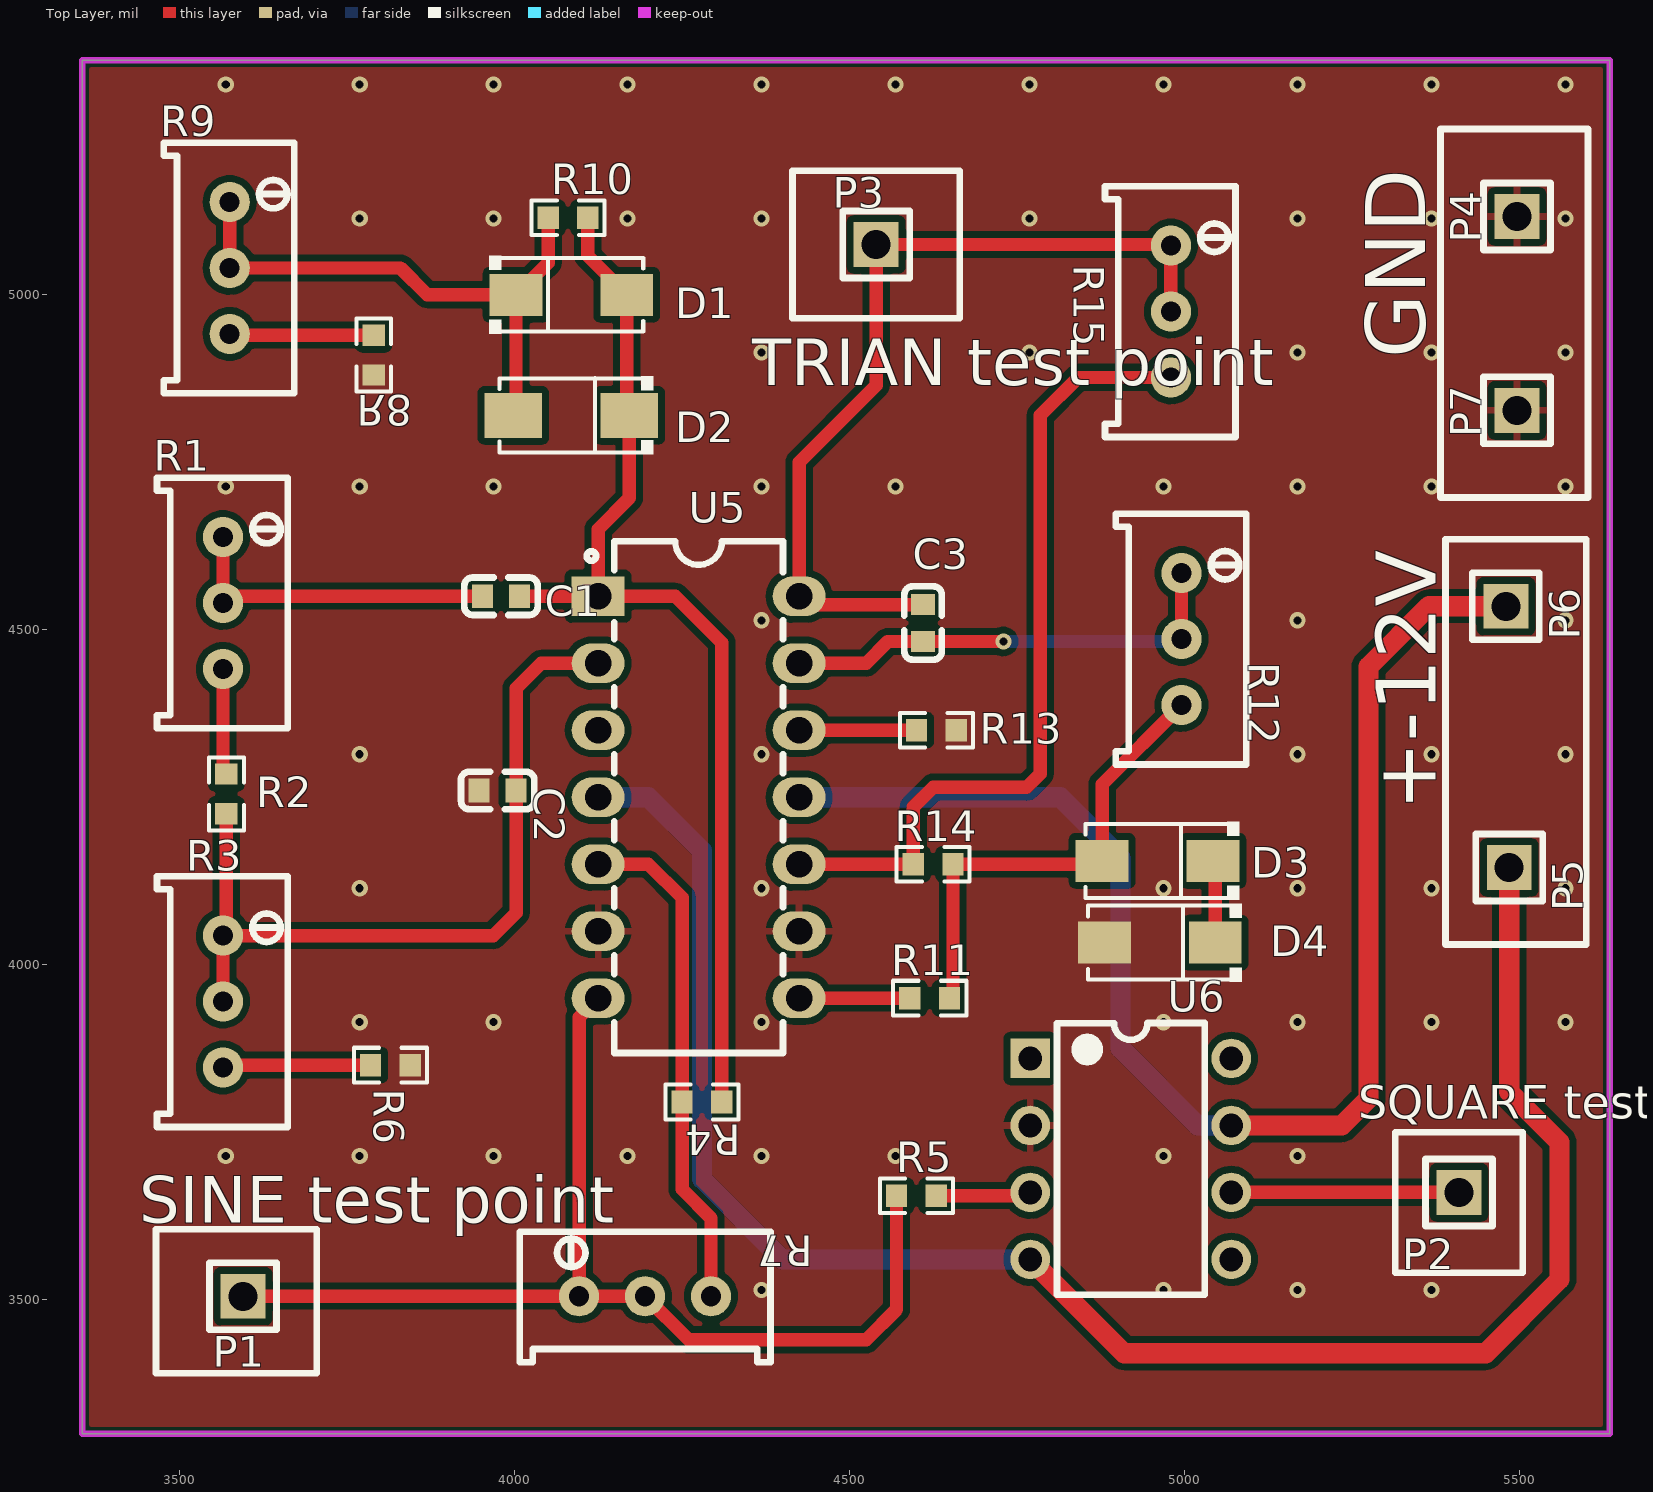
[diagram p0: Top Layer view]
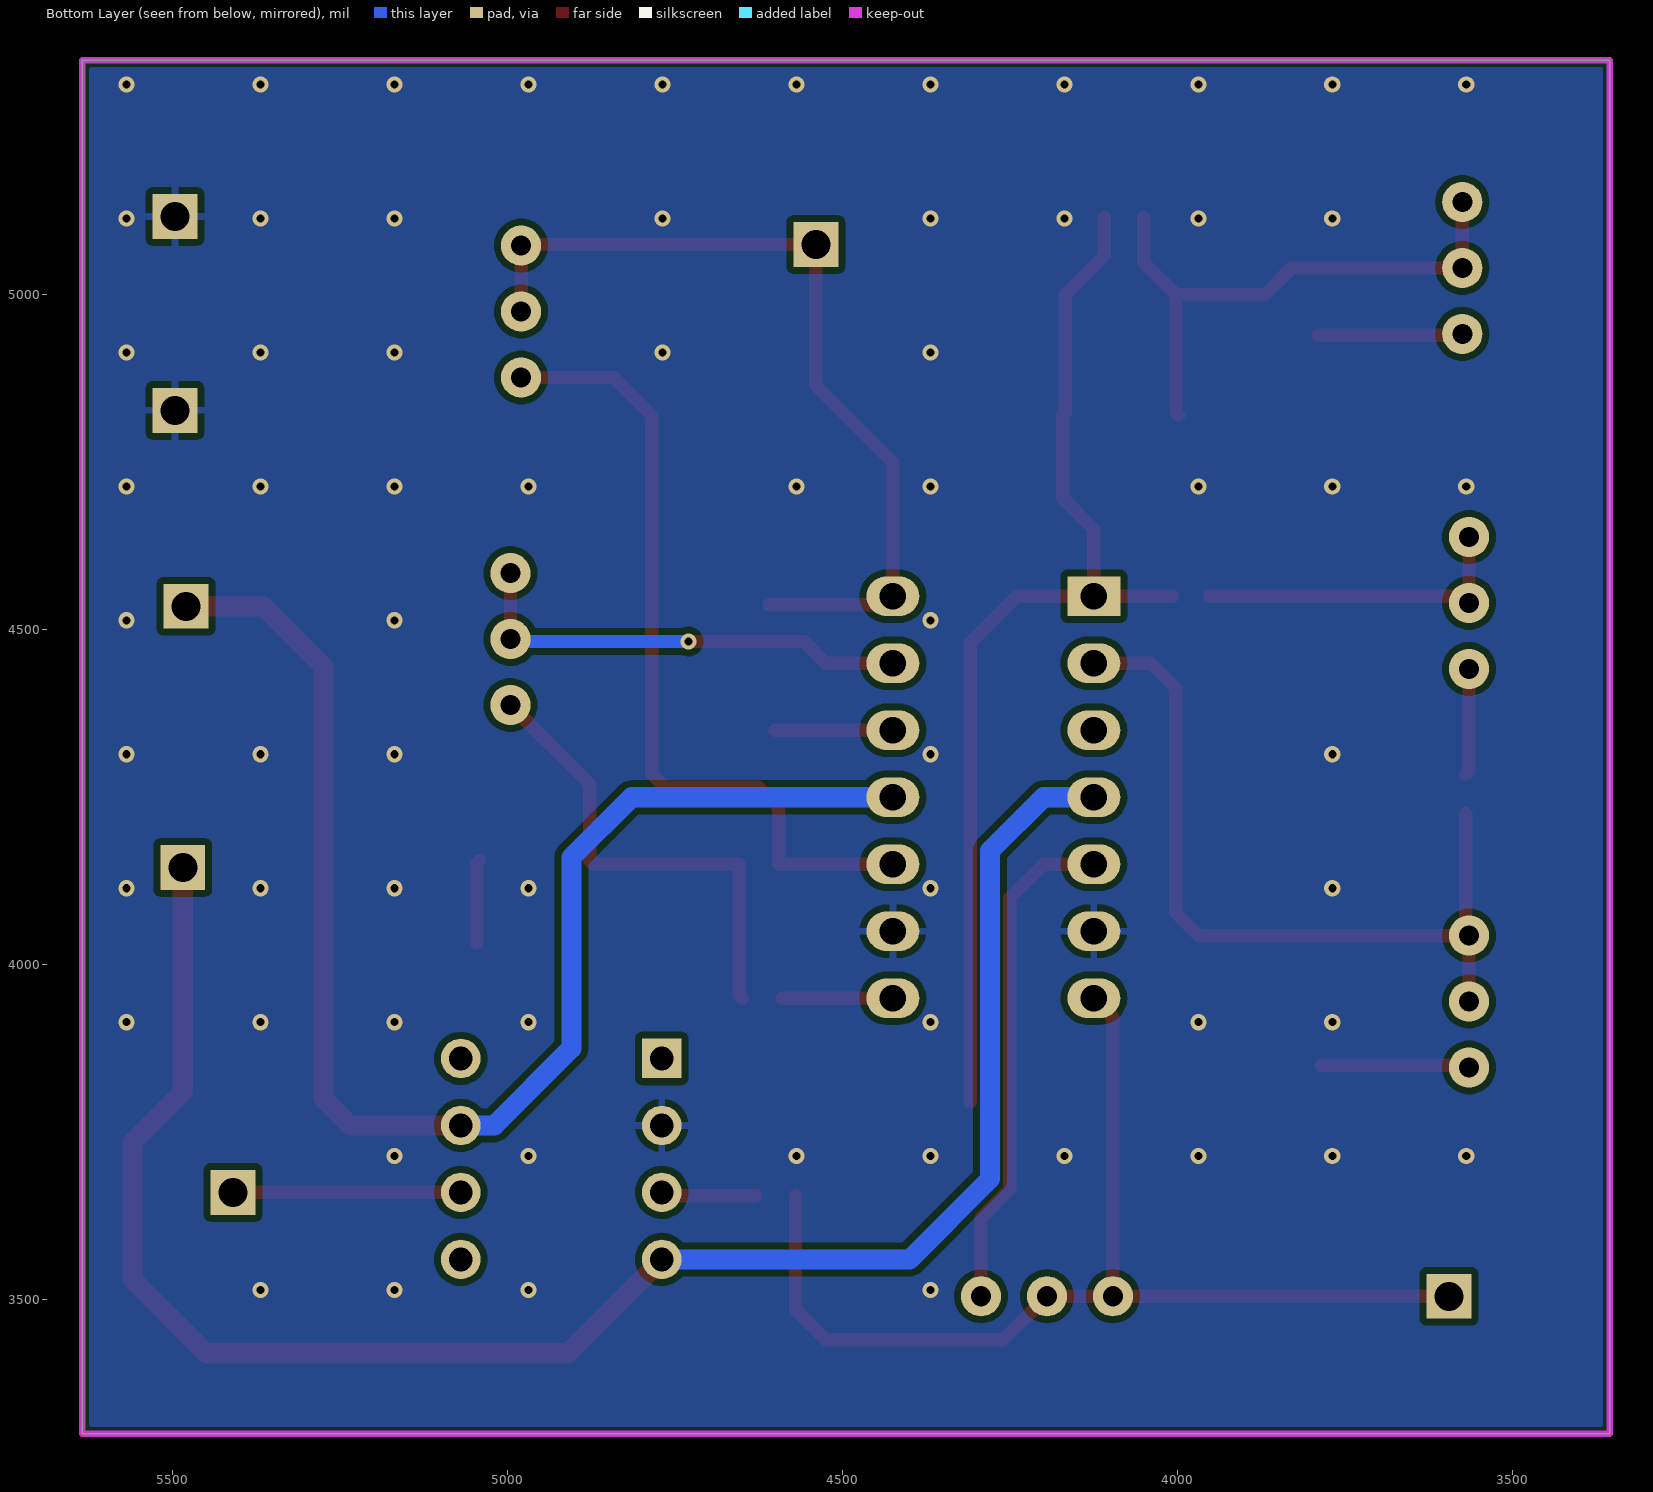
[diagram p1: Bottom Layer view, seen from below]
# Altium PCB MISC51008.pcbdoc
Units mil, origin at the board's own origin, x right, y up, seen from the top; angles counter-clockwise.
Board outline 2280 x 2050 mil, 2 copper layers (Top Layer, Bottom Layer), stack 62.206 mil thick; 31 components, 21 nets, 79 pads, 67 vias.

## Layer stack, top to bottom
Top Solder Mask Layer: solder mask 0.394, Dk 3.3
Top Layer: signal copper 1.379
Dielectric1: surface 59.449, FR4, Dk 4.5
Bottom Layer: signal copper 1.378
Bottom Solder Mask Layer: solder mask 0.394, Dk 3.3

## Board outline
3355,5350 3355,3300 5635,3300 5635,5350

## Design rules (kind name [scope] priority, off if disabled: settings)
BoardOutlineClearance copperThickness2oz_1 [All] p2 off: genericclearance=7.99 ignorepadtopadclearanceinfootprint=FALSE except(0: Arc-SplitContinuation Track-SplitContinuation SMDPad-SplitContinuation THPad-SplitContinuation Via-SplitContinuation Fill-SplitContinuation Region-SplitContinuation Poly-SplitContinuation Text-SplitContinuation Hole-SplitContinuation; 5.98: Arc-CutoutEdge SMDPad-CutoutEdge THPad-CutoutEdge Via-CutoutEdge Fill-CutoutEdge Region-CutoutEdge Text-CutoutEdge; 6.93: Hole-OutlineEdge Hole-CutoutEdge; 10: Poly-OutlineEdge Poly-CutoutEdge; 11.81: Arc-OutlineEdge Track-OutlineEdge SMDPad-OutlineEdge THPad-OutlineEdge Via-OutlineEdge Fill-OutlineEdge Region-OutlineEdge Text-OutlineEdge Track-CutoutEdge)
BoardOutlineClearance Plane_innerPlane_1 [All] p4 off: genericclearance=4.02 ignorepadtopadclearanceinfootprint=FALSE except(0: Arc-SplitContinuation Track-SplitContinuation SMDPad-SplitContinuation THPad-SplitContinuation Via-SplitContinuation Fill-SplitContinuation Region-SplitContinuation Poly-SplitContinuation Text-SplitContinuation Hole-SplitContinuation; 5.98: SMDPad-CutoutEdge THPad-CutoutEdge Via-CutoutEdge Fill-CutoutEdge Region-CutoutEdge Text-CutoutEdge; 6.93: Hole-OutlineEdge Hole-CutoutEdge; 10: Poly-OutlineEdge Poly-CutoutEdge; 11.81: Arc-OutlineEdge Track-OutlineEdge SMDPad-OutlineEdge THPad-OutlineEdge Via-OutlineEdge Fill-OutlineEdge Region-OutlineEdge Text-OutlineEdge Arc-CutoutEdge Track-CutoutEdge)
BoardOutlineClearance Copper_copperRegion_1 [All] p6 off: genericclearance=4.02 ignorepadtopadclearanceinfootprint=FALSE except(0: Arc-SplitContinuation Track-SplitContinuation SMDPad-SplitContinuation THPad-SplitContinuation Via-SplitContinuation Fill-SplitContinuation Region-SplitContinuation Poly-SplitContinuation Text-SplitContinuation Hole-SplitContinuation; 5.98: SMDPad-CutoutEdge THPad-CutoutEdge Via-CutoutEdge Fill-CutoutEdge Region-CutoutEdge Text-CutoutEdge; 6.93: Hole-OutlineEdge Hole-CutoutEdge; 10: Poly-OutlineEdge Poly-CutoutEdge; 11.81: Arc-OutlineEdge Track-OutlineEdge SMDPad-OutlineEdge THPad-OutlineEdge Via-OutlineEdge Fill-OutlineEdge Region-OutlineEdge Text-OutlineEdge Arc-CutoutEdge Track-CutoutEdge)
BoardOutlineClearance copperThickness1oz_1 [All] p8: genericclearance=4.02 ignorepadtopadclearanceinfootprint=FALSE except(0: Arc-SplitContinuation Track-SplitContinuation SMDPad-SplitContinuation THPad-SplitContinuation Via-SplitContinuation Fill-SplitContinuation Region-SplitContinuation Poly-SplitContinuation Text-SplitContinuation Hole-SplitContinuation; 5.98: SMDPad-CutoutEdge THPad-CutoutEdge Via-CutoutEdge Fill-CutoutEdge Region-CutoutEdge Text-CutoutEdge; 6.93: Hole-OutlineEdge Hole-CutoutEdge; 10: Poly-OutlineEdge Poly-CutoutEdge; 11.81: Arc-OutlineEdge Track-OutlineEdge SMDPad-OutlineEdge THPad-OutlineEdge Via-OutlineEdge Fill-OutlineEdge Region-OutlineEdge Text-OutlineEdge Arc-CutoutEdge Track-CutoutEdge)
Clearance copperThickness2oz [All] p1 off: gap=7.99 ignorepadtopadclearanceinfootprint=FALSE except(5.98: SMDPad-Track SMDPad-SMDPad THPad-Track SMDPad-THPad THPad-THPad Track-Via SMDPad-Via THPad-Via Via-Via Fill-Track Region-Track Fill-SMDPad Region-SMDPad Fill-THPad Region-THPad Fill-Via Region-Via Fill-Fill Fill-Region Region-Region Arc-Track Arc-SMDPad Arc-THPad Arc-Via Fill-Arc Region-Arc Arc-Arc Text-Track SMDPad-Text Text-THPad Text-Via Fill-Text Region-Text Arc-Text Text-Text; 6.93: Hole-Track Hole-SMDPad Hole-THPad Hole-Via Fill-Hole Region-Hole Hole-Arc Hole-Text; 10: Poly-Track Poly-SMDPad Poly-THPad Poly-Via Poly-Fill Poly-Region Poly-Poly Poly-Arc Poly-Text Poly-Hole)
Clearance Plane_innerPlane [All] p3 off: gap=4.02 ignorepadtopadclearanceinfootprint=FALSE except(5.98: SMDPad-Track SMDPad-SMDPad THPad-Track SMDPad-THPad THPad-THPad Track-Via SMDPad-Via THPad-Via Via-Via Fill-Track Region-Track Fill-SMDPad Region-SMDPad Fill-THPad Region-THPad Fill-Via Region-Via Fill-Fill Fill-Region Region-Region Arc-Track Arc-SMDPad Arc-THPad Arc-Via Fill-Arc Region-Arc Arc-Arc Text-Track SMDPad-Text Text-THPad Text-Via Fill-Text Region-Text Arc-Text Text-Text; 6.93: Hole-Track Hole-SMDPad Hole-THPad Hole-Via Fill-Hole Region-Hole Hole-Arc Hole-Text; 10: Poly-Track Poly-SMDPad Poly-THPad Poly-Via Poly-Fill Poly-Region Poly-Poly Poly-Arc Poly-Text Poly-Hole)
Clearance Copper_copperRegion [All] p5 off: gap=4.02 ignorepadtopadclearanceinfootprint=FALSE except(5.98: SMDPad-Track SMDPad-SMDPad THPad-Track SMDPad-THPad THPad-THPad Track-Via SMDPad-Via THPad-Via Via-Via Fill-Track Region-Track Fill-SMDPad Region-SMDPad Fill-THPad Region-THPad Fill-Via Region-Via Fill-Fill Fill-Region Region-Region Arc-Track Arc-SMDPad Arc-THPad Arc-Via Fill-Arc Region-Arc Arc-Arc Text-Track SMDPad-Text Text-THPad Text-Via Fill-Text Region-Text Arc-Text Text-Text; 6.93: Hole-Track Hole-SMDPad Hole-THPad Hole-Via Fill-Hole Region-Hole Hole-Arc Hole-Text; 10: Poly-Track Poly-SMDPad Poly-THPad Poly-Via Poly-Fill Poly-Region Poly-Poly Poly-Arc Poly-Text Poly-Hole)
Clearance copperThickness1oz [All] p7: gap=4.02 ignorepadtopadclearanceinfootprint=FALSE except(5.98: SMDPad-Track SMDPad-SMDPad THPad-Track SMDPad-THPad THPad-THPad Track-Via SMDPad-Via THPad-Via Via-Via Fill-Track Region-Track Fill-SMDPad Region-SMDPad Fill-THPad Region-THPad Fill-Via Region-Via Fill-Fill Fill-Region Region-Region Arc-Track Arc-SMDPad Arc-THPad Arc-Via Fill-Arc Region-Arc Arc-Arc Text-Track SMDPad-Text Text-THPad Text-Via Fill-Text Region-Text Arc-Text Text-Text; 6.93: Hole-Track Hole-SMDPad Hole-THPad Hole-Via Fill-Hole Region-Hole Hole-Arc Hole-Text; 10: Poly-Track Poly-SMDPad Poly-THPad Poly-Via Poly-Fill Poly-Region Poly-Poly Poly-Arc Poly-Text Poly-Hole)
DiffPairsRouting differentialPair [All] p1: maxlimit=6 minlimit=6 mostfreqgap=6 toplayer_minwidth=5 toplayer_prefwidth=10 toplayer_maxwidth=100 toplayer_mingap=6 toplayer_prefgap=6 toplayer_maxgap=6 bottomlayer_minwidth=5 bottomlayer_prefwidth=10 bottomlayer_maxwidth=100 bottomlayer_mingap=6 bottomlayer_prefgap=6 bottomlayer_maxgap=6 maxuncoupledlength=10
HoleToHoleClearance otherClearance [All] p1: gap=11.81 allowstackedmicrovias=TRUE
Length netLength [All] p1: minlimit=0 maxlimit=0
PasteMaskExpansion pasteMaskExpansion [All] p1: expansion=0
PlaneConnect innerPlane [All] p1: planeconnectstyle=Relief reliefexpansion=20 reliefentries=4 reliefconductorwidth=10 reliefairgap=10
PolygonConnect copperRegion [All] p1: connectstyle=Relief reliefconductorwidth=10 reliefentries=4 polygonreliefangle="90 Angle" airgapwidth=10 smdpad.connectstyle=Direct via.connectstyle=Relief via.reliefconductorwidth=10 via.reliefentries=4 via.polygonreliefangle="90 Angle" via.airgapwidth=10
RoutingVias viaSize [All] p1: holewidth=12.01 width=24.02 viastyle="Through Hole" minholewidth=11.81 minwidth=19.68 maxholewidth=248.03 maxwidth=393.7
SolderMaskExpansion solderMaskExpansion [IsVia] p1: expansion=-1000 istentingtop=TRUE
SolderMaskExpansion solderMaskExpansion [All] p2: expansion=2.01 istentingtop=FALSE
Width copperThickness2oz_2 [All] p1 off: maxlimit=100 minlimit=8 preferedwidth=10
Width copperThickness1oz_2 [All] p2: maxlimit=100 minlimit=5 preferedwidth=10

## Components (designator, comment, footprint, x,y, rotation, side; value= is the part's Value field where it differs from the comment)
C1 "100nF" C0603 3980,4550 r0 top
C2 "100nF" C0603 3975,4260 r0 top
C3 "100nF" C0603 4610,4510 r90 top
D1 "1N4007" SMA_L4.3-W2.5-LS5.0-RD 4085,5000 r0 top
D2 "1N4007" SMA_L4.3-W2.5-LS5.0-RD-1 4085,4820 r180 top
D3 "1N4007" SMA_L4.3-W2.5-LS5.0-RD 4960,4155 r180 top
D4 "1N4007" SMA_L4.3-W2.5-LS5.0-RD 4963.42,4032.83 r180 top
P1 "2.54-1*1P pin" HDR-TH_1P-P2.54-V-M 3595,3505 r0 top
P2 "2.54-1*1P pin" HDR-TH_1P-P2.54-V-M 5410,3660 r0 top
P3 "2.54-1*1P pin" HDR-TH_1P-P2.54-V-M 4540,5075 r0 top
P4 "2.54-1*1P pin" HDR-TH_1P-P2.54-V-M 5496.62,5116.89 r90 top
P5 "2.54-1*1P pin" HDR-TH_1P-P2.54-V-M 5485,4145 r90 top
P6 "2.54-1*1P pin" HDR-TH_1P-P2.54-V-M 5480,4535 r90 top
P7 "2.54-1*1P pin" HDR-TH_1P-P2.54-V-M 5496.62,4827.5 r90 top
R1 "50kΩ" RES-ADJ-TH_3P-L9.5-W4.85-P2.50-BL-BS 3565,4540 r0 top
R2 "5.1kΩ" R0603 3570,4255 r90 top
R3 "50kΩ" RES-ADJ-TH_3P-L9.5-W4.85-P2.50-BL-BS 3565,3945 r0 top
R4 "200Ω" R0603 4280,3795 r180 top
R5 "20kΩ" R0603 4600,3655 r0 top
R6 "5.1kΩ" R0603 3815,3850 r180 top
R7 "50kΩ" RES-ADJ-TH_3P-L9.5-W4.85-P2.50-BL-BS 4195,3505 r90 top
R8 "5.1kΩ" R0603 3790,4910 r90 top
R9 "50kΩ" RES-ADJ-TH_3P-L9.5-W4.85-P2.50-BL-BS 3575,5040 r0 top
R10 "5.1kΩ" R0603 4080,5115 r0 top
R11 "5.1kΩ" R0603 4620,3950 r0 top
R12 "50kΩ" RES-ADJ-TH_3P-L9.5-W4.85-P2.50-BL-BS 4995.88,4486.09 r0 top
R13 "5.1kΩ" R0603 4630,4350 r180 top
R14 "5.1kΩ" R0603 4625,4150 r0 top
R15 "50kΩ" RES-ADJ-TH_3P-L9.5-W4.85-P2.50-BL-BS 4980,4975 r0 top
U5 "LM324N" DIP-14_L19.4-W6.4-P2.54-LS7.6-BL 4275,4250 r270 top
U6 "LM741J" CDIP-8_L10.3-W6.7-P2.54-LS7.6-BL 4920,3710 r270 top

## Footprints (in the part's own frame and the unit in brackets; to place one, negate y for a bottom-side part, rotate by r counter-clockwise, add the part's x,y. Pads: shape width x height; smd on the part's side, far side on the other; paste and mask are expansions set on the pad)
C0603 [mm]
  rect 0.8x0.9 smd: 1(-0.7,0) 2(0.7,0)
  silkscreen extent -1.39,-0.71 1.39,0.71
CDIP-8_L10.3-W6.7-P2.54-LS7.6-BL [mm]
  rect 1.5x1.5 hole 0.9: 1(-3.81,-3.81)
  round 1.5 hole 0.9: 2(-1.27,-3.81) 3(1.27,-3.81) 4(3.81,-3.81) 5(3.81,3.81) 6(1.27,3.81) 7(-1.27,3.81) 8(-3.81,3.81)
  silkscreen extent -5.15,-2.79 5.15,2.81
DIP-14_L19.4-W6.4-P2.54-LS7.6-BL [mm]
  rect 1.5x2 hole 1: 1(-7.62,-3.811)
  oval 1.5x2 hole 1: 2(-5.08,-3.811) 3(-2.54,-3.811) 4(0,-3.811) 5(2.54,-3.811) 6(5.08,-3.811) 7(7.62,-3.811) 8(7.62,3.811) 9(5.08,3.809) 10(2.54,3.809) 11(0,3.809) 12(-2.54,3.809) 13(-5.08,3.809) 14(-7.62,3.809)
  silkscreen extent -9.7,-4.24 9.7,3.2
HDR-TH_1P-P2.54-V-M [mm]
  rect 1.7x1.7 hole 1.1: 1(0,0)
  silkscreen extent -1.27,-1.27 1.27,1.27
R0603 [mil]
  rect 31.75x34.02 smd paste-3937.01 mask+2: 1(-29.66,0) 2(29.66,0)
  silkscreen extent -55,-26 55,26
RES-ADJ-TH_3P-L9.5-W4.85-P2.50-BL-BS [mil]
  round 60 hole 30: 1(0,98.43) 2(0,0) 3(0,-98.43)
  silkscreen extent -98,-187 96,187
SMA_L4.3-W2.5-LS5.0-RD [mm]
  rect 2x1.593 smd: 1(-2.1,0) 2(2.1,0)
  silkscreen extent -3.11,-1.48 2.73,1.48
SMA_L4.3-W2.5-LS5.0-RD-1 [mm]
  rect 2.185x1.7 smd: 1(-2.2,0) 2(2.2,0)
  silkscreen extent -3.11,-1.48 2.73,1.48

## Via types
v1: diameter 24.02, hole 12, Top Layer to Bottom Layer, 67 vias

## Nets (pads, with @x,y where several pads share a name; then routed paths per layer and width w, separated by ;. In a path a pad name is that pad's centre, name@x,y a point inside that pad or via, vN(x,y) a via of type N, cw(c..) or ccw(c..) an arc to the next point about the centre after c; other vN are vias at no path point)
$1N8: C2.2 R2.1 R3.1 R3.2 U5.2 | length 1207
  Top Layer w20: R3.2 R3.1 ; R2.1 3570,4048.43 R3.1 ; U5.2 4040,4450 4002.56,4412.56 C2.2 4002.56,4077.56 3968.43,4043.43 R3.1
$1N11: R3.3 R6.2 | length 221.8
  Top Layer w20: R3.3 3568.43,3850 R6.2
$1N12: R8.2 R9.3 | length 215.8
  Top Layer w20: R9.3 3576.91,4939.66 R8.2
$1N13: D1.1 D2.2 R9.1 R9.2 R10.1 | length 858.8
  Top Layer w20: R9.1 R9.2 3830.01,5039.99 3870,5000 D1.1 ; D2.2 4002.32,4823.94 D1.1 ; R10.1 4050.34,5048.02 D1.1
$1N14: R1.3 R2.2 | length 159
  Top Layer w20: R1.3 3565,4289.66 R2.2
$1N15: C1.1 R1.1 R1.2 | length 490
  Top Layer w20: R1.1 R1.2 3575.01,4550 C1.1
$1N18: C1.2 D1.2 D2.1 R4.1 R10.2 U5.1 | length 1626.3
  Top Layer w20: C1.2 U5.1 ; R10.2 4109.66,5058.02 D1.2 4167.68,4823.94 D2.1 4171.61,4696.61 4124.98,4649.98 U5.1 ; R4.1 4309.66,4480.34 4240,4550 U5.1
$1N23: R4.2 R7.3 U5.5 | length 758.7
  Top Layer w20: U5.5 4200,4150 4250.34,4099.66 R4.2 4250.34,3664.66 4293.43,3621.57 R7.3
$1N26: R11.1 U5.8 | length 165.3
  Top Layer w20: U5.8 R11.1
$1N27: D3.2 R11.2 R12.3 R14.2 | length 708.6
  Top Layer w20: R11.2 4654.66,3955 R14.2 4872.32,4150 D3.2 4877.32,4269.1 R12.3
$1N28: C3.1 R12.1 R12.2 U5.13 | length 684.3
  Top Layer w20: U5.13 4525,4450 4557.44,4482.44 C3.1 v1(4730,4482.44) ; R12.2 R12.1
  Bottom Layer w20: v1(4730,4482.44) 4992.23,4482.44 R12.2
$1N29: R14.1 R15.3 U5.10 | length 1219.4
  Top Layer w20: U5.10 R14.1 4595.34,4235.34 4625,4265 4765,4265 4785,4285 4785,4820 4841.57,4876.57 R15.3
$1N32: D3.1 D4.1 | length 123.6
  Top Layer w20: D3.1 5046.1,4151.58 D4.1
$1N36: R13.2 U5.12 | length 175.4
  Top Layer w20: U5.12 R13.2
$1N39: R5.2 U6.3 | length 142.4
  Top Layer w20: R5.2 4765,3655 U6.3
+12V: P6.1 U5.11 U6.7 | length 2123.8
  Top Layer w30: U6.7 5235,3760 5275,3800 5275,4445 5365,4535 P6.1
  Bottom Layer w30: U5.11 4815,4250 4905,4160 4905,3875 5020,3760 U6.7
-12V: P5.1 U5.4 U6.4 | length 2757.5
  Top Layer w30: U6.4 4910,3420 5450,3420 5560,3530 5560,3735 5485,3810 P5.1
  Bottom Layer w30: U5.4 4200,4250 4280,4170 4280,3680 4400,3560 U6.4
GND: C2.1 D4.2 P4.1 P7.1 R6.1 R8.1 R13.1 U5.6 U5.9 U6.2
  other v1: 4369.1,3514.1 4969.1,3514.1 5169.1,3514.1 5369.1,3514.1 3569.1,3714.1 3769.1,3714.1 3969.1,3714.1 4169.1,3714.1 4369.1,3714.1 4569.1,3714.1 4969.1,3714.1 5169.1,3714.1 3769.1,3914.1 3969.1,3914.1 4369.1,3914.1 4969.1,3914.1 5169.1,3914.1 5369.1,3914.1 5569.1,3914.1 3769.1,4114.1 4369.1,4114.1 4969.1,4114.1 5169.1,4114.1 5369.1,4114.1 5569.1,4114.1 3769.1,4314.1 4369.1,4314.1 5169.1,4314.1 5369.1,4314.1 5569.1,4314.1 4369.1,4514.1 5169.1,4514.1 5569.1,4514.1 3569.1,4714.1 3769.1,4714.1 3969.1,4714.1 4369.1,4714.1 4569.1,4714.1 4969.1,4714.1 5169.1,4714.1 5369.1,4714.1 5569.1,4714.1 4369.1,4914.1 4769.1,4914.1 5169.1,4914.1 5369.1,4914.1 5569.1,4914.1 3769.1,5114.1 3969.1,5114.1 4169.1,5114.1 4369.1,5114.1 4769.1,5114.1 5169.1,5114.1 5369.1,5114.1 5569.1,5114.1 3569.1,5314.1 3769.1,5314.1 3969.1,5314.1 4169.1,5314.1 4369.1,5314.1 4569.1,5314.1 4769.1,5314.1 4969.1,5314.1 5169.1,5314.1 5369.1,5314.1 5569.1,5314.1
SINE: P1.1 R5.1 R7.1 R7.2 U5.7 | length 1647.5
  Top Layer w20: P1.1 R7.1 ; U5.7 4096.57,3921.59 R7.1 ; R5.1 4570.34,3485.34 4525,3440 4260.01,3440 R7.2 R7.1
SQUARE: P2.1 U6.6 | length 340
  Top Layer w20: U6.6 P2.1
TRIAN: C3.2 P3.1 R15.1 R15.2 U5.14 | length 1301.9
  Top Layer w20: C3.2 4437.42,4537.56 U5.14 4424.98,4749.98 4540,4865 P3.1 4978.43,5075 R15.1 R15.2
pads on no net: U5.3 U6.1 U6.5 U6.8

## Polygon pours and split planes (outlines as drawn)
GND on Top Layer (solid, remove dead copper, pour order 0): 3000,5495 3000,3000 6340,3000 6340,5495
GND on Bottom Layer (solid, remove dead copper, pour order 2): 3345,5525 3345,3065 6455,3065 6455,5525

## Keep-outs
Board Outline Layer:
  the board outline again, w10

## Silkscreen, mask and mechanical layers (free items; w line width, h text height)
Top Silkscreen Layer:
  lines w10: 3465,3390 3465,3605 3705,3605 3705,3390 3465,3390 ; 4415,4965 4415,5185 4665,5185 4665,4965 4415,4965 ; 5315,3540 5315,3750 5505,3750 5505,3540 5315,3540 ; 5382.5,4697.5 5602.5,4697.5 5602.5,5247.5 5382.5,5247.5 5382.5,4697.5 ; 5390,4030 5600,4030 5600,4635 5390,4635 5390,4030
  text "GND" at 5360,4905 h90 r90
  text "TRIAN test point" at 4355,4865 h70
  text "+-12V" at 5375,4230 h90 r90
  text "SQUARE test point" at 5260,3770 h50
  text "SINE test point" at 3440,3615 h70